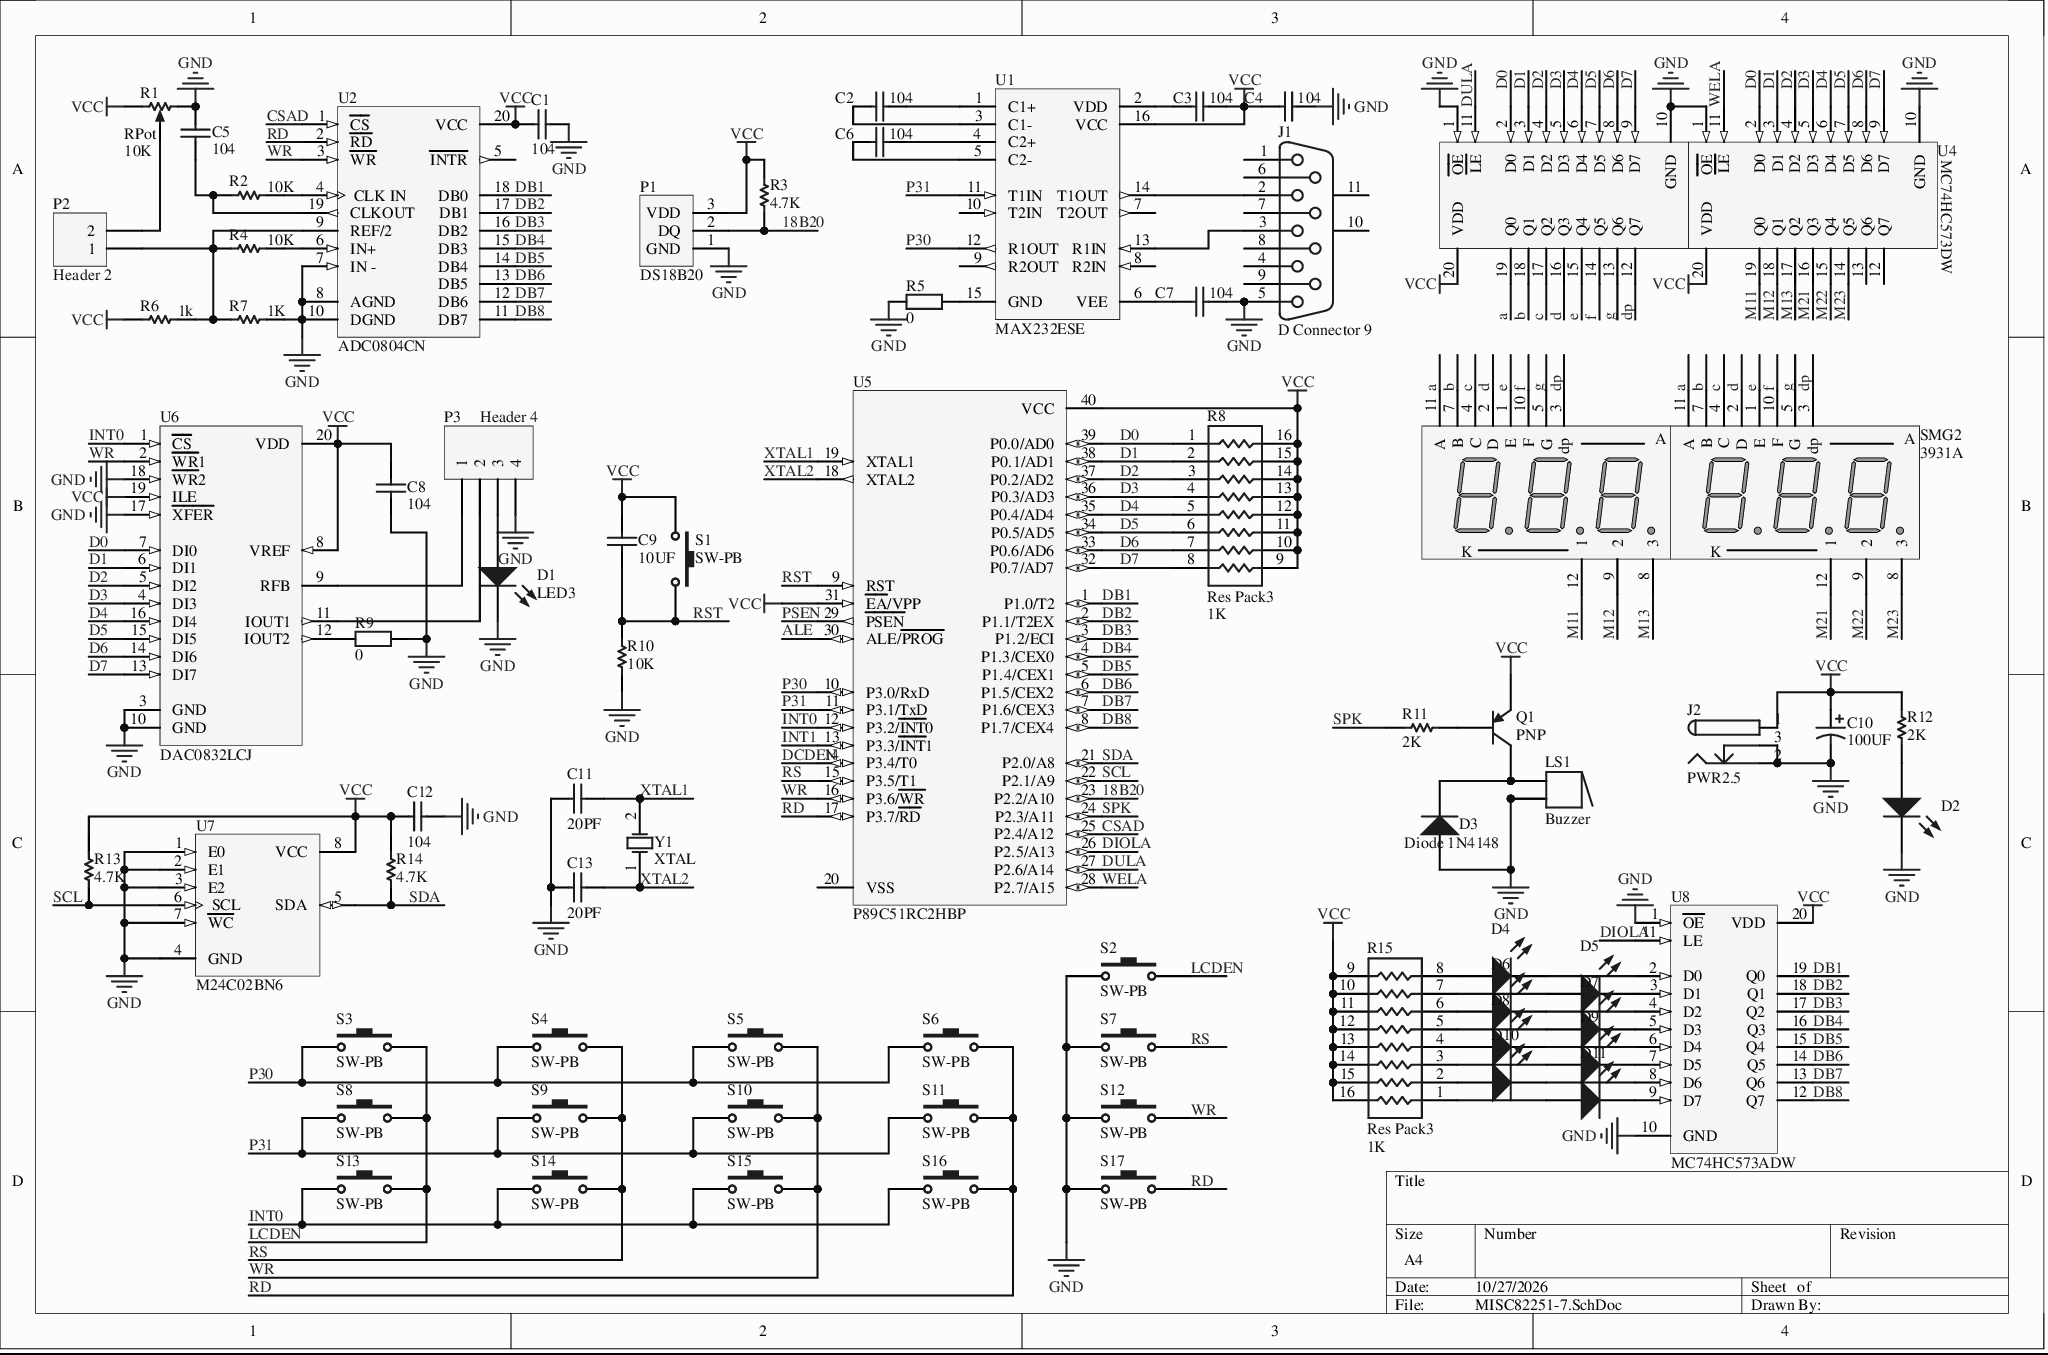
[diagram p0: MISC82251-7.SchDoc]
# Altium project MISC82251-3.PrjPcb
1 sheet, 74 parts. Net scope: global (net labels, ports and power ports of the same name join across sheets).
Board file: MISC82251.PcbDoc

## Sheet MISC82251-7.SchDoc
size A4

### Parts
C1  104  [RAD-0.3]
C2  104  [RAD-0.3]
C3  104  [RAD-0.3]
C4  104  [RAD-0.3]
C5  104  [RAD-0.3]
C6  104  [RAD-0.3]
C7  104  [RAD-0.3]
C8  104  [RAD-0.3]
C9  10UF  [RAD-0.3]
C10  100UF  [RB7.6-15]
C11  20PF  [RAD-0.1]
C12  104  [RAD-0.3]
C13  20PF  [RAD-0.1]
D1  LED3  [3.5X2.8X1.9]
D2  LED3  [3.5X2.8X1.9]  (value not drawn)
D3  Diode 1N4148  [DO-35]
D4  LED3  [3.5X2.8X1.9]  (value not drawn)
D5  LED3  [3.5X2.8X1.9]  (value not drawn)
D6  LED3  [3.5X2.8X1.9]  (value not drawn)
D7  LED3  [3.5X2.8X1.9]  (value not drawn)
D8  LED3  [3.5X2.8X1.9]  (value not drawn)
D9  LED3  [3.5X2.8X1.9]  (value not drawn)
D10  LED3  [3.5X2.8X1.9]  (value not drawn)
D11  LED3  [3.5X2.8X1.9]  (value not drawn)
J1  D Connector 9  [DSUB1.385-2H9]
J2  PWR2.5  [DC-002]
LS1  Buzzer  [ABSM-1574]
P1  DS18B20  [HDR1X3]
P2  Header 2  [HDR1X2]
P3  Header 4  [HDR1X4]
Q1  PNP  [SOT-23B_N]
R1  RPot  value 10K  [VR5]
R2  10K  [AXIAL-0.3]
R3  4.7K  [AXIAL-0.3]
R4  10K  [AXIAL-0.3]
R5  0  [AXIAL-0.4]
R6  1k  [AXIAL-0.3]
R7  1K  [AXIAL-0.3]
R8  Res Pack3  value 1K  [SO-16_N]
R9  0  [AXIAL-0.4]
R10  10K  [AXIAL-0.3]
R11  2K  [AXIAL-0.3]
R12  2K  [AXIAL-0.3]
R13  4.7K  [AXIAL-0.3]
R14  4.7K  [AXIAL-0.3]
R15  Res Pack3  value 1K  [SO-16_N]
S1  SW-PB  [SPST-2]
S2  SW-PB  [SPST-2]
S3  SW-PB  [SPST-2]
S4  SW-PB  [SPST-2]
S5  SW-PB  [SPST-2]
S6  SW-PB  [SPST-2]
S7  SW-PB  [SPST-2]
S8  SW-PB  [SPST-2]
S9  SW-PB  [SPST-2]
S10  SW-PB  [SPST-2]
S11  SW-PB  [SPST-2]
S12  SW-PB  [SPST-2]
S13  SW-PB  [SPST-2]
S14  SW-PB  [SPST-2]
S15  SW-PB  [SPST-2]
S16  SW-PB  [SPST-2]
S17  SW-PB  [SPST-2]
SMG1  3931A  [SMG 0.39-3P]
SMG2  3931A  [SMG 0.39-3P]
U1  MAX232ESE  [DIP16]
U2  ADC0804CN  [N020]
U3  MC74HC573DW  [751D-03]
U4  MC74HC573DW  [751D-03]
U5  P89C51RC2HBP  [SOT129-1]
U6  DAC0832LCJ  [J20A]
U7  M24C02BN6  [PSDIP8A]
U8  MC74HC573ADW  [751D-05]
Y1  XTAL  [R38]

### Nets
GND: C1.1 C4.1 C5.2 C7.1 C8.2 C10.2 C11.2 C12.2 C13.2 D1.2(K) D2.2(K) D3.1(A) J1.5 J2.2 J2.3 LS1.2 LS1.2A P1.1(GND) P3.4 R1.2(BOT) R5.1 R7.2 R9.2 R10.1 S2.1 S7.1 S12.1 S17.1 U2.7(IN_-) U2.8(AGND) U2.10(DGND) U3.1(~{OE}) U3.10(GND) U4.1(~{OE}) U4.10(GND) U6.3(GND) U6.10(GND) U6.17(~{XFER}) U6.18(~{WR}2) U7.1(E0) U7.2(E1) U7.3(E2) U7.4(GND) U7.7(~{WC}) U8.1(~{OE}) U8.10(GND)
VCC: C1.2 C3.1 C4.2 C8.1 C9.2 C10.1 C12.1 J2.1 P1.3(VDD) Q1.3(E) R1.1(TOP) R3.2 R6.1 R8.9 R8.10 R8.11 R8.12 R8.13 R8.14 R8.15 R8.16 R12.2 R13.2 R14.2 R15.9 R15.10 R15.11 R15.12 R15.13 R15.14 R15.15 R15.16 S1.1 U1.16(VCC) U2.20(VCC) U3.20(VDD) U4.20(VDD) U5.31(~{EA}/VPP) U5.40(VCC) U6.8(VREF) U6.19(ILE) U6.20(VDD) U7.8(VCC) U8.20(VDD)
18B20: P1.2(DQ) R3.1 U5.23(P2.2/A10)
a: SMG1.11(A) SMG2.11(A) U3.19(Q0)
ALE: U5.30(ALE/~{PROG})
b: SMG1.7(B) SMG2.7(B) U3.18(Q1)
c: SMG1.4(C) SMG2.4(C) U3.17(Q2)
CSAD: U2.1(~{CS}) U5.25(P2.4/A12)
d: SMG1.2(D) SMG2.2(D) U3.16(Q3)
D0: R8.1 U3.2(D0) U4.2(D0) U5.39(P0.0/AD0) U6.7(DI0)
D1: R8.2 U3.3(D1) U4.3(D1) U5.38(P0.1/AD1) U6.6(DI1)
D2: R8.3 U3.4(D2) U4.4(D2) U5.37(P0.2/AD2) U6.5(DI2)
D3: R8.4 U3.5(D3) U4.5(D3) U5.36(P0.3/AD3) U6.4(DI3)
D4: R8.5 U3.6(D4) U4.6(D4) U5.35(P0.4/AD4) U6.16(DI4)
D5: R8.6 U3.7(D5) U4.7(D5) U5.34(P0.5/AD5) U6.15(DI5)
D6: R8.7 U3.8(D6) U4.8(D6) U5.33(P0.6/AD6) U6.14(DI6)
D7: R8.8 U3.9(D7) U4.9(D7) U5.32(P0.7/AD7) U6.13(DI7)
DB1: U2.18(DB0) U5.1(P1.0/T2) U8.19(Q0)
DB2: U2.17(DB1) U5.2(P1.1/T2EX) U8.18(Q1)
DB3: U2.16(DB2) U5.3(P1.2/ECI) U8.17(Q2)
DB4: U2.15(DB3) U5.4(P1.3/CEX0) U8.16(Q3)
DB5: U2.14(DB4) U5.5(P1.4/CEX1) U8.15(Q4)
DB6: U2.13(DB5) U5.6(P1.5/CEX2) U8.14(Q5)
DB7: U2.12(DB6) U5.7(P1.6/CEX3) U8.13(Q6)
DB8: U2.11(DB7) U5.8(P1.7/CEX4) U8.12(Q7)
DCDEN: U5.14(P3.4/T0)
DIOLA: U5.26(P2.5/A13) U8.11(LE)
dp: SMG1.3(dp) SMG2.3(dp) U3.12(Q7)
DULA: U3.11(~{LE}) U5.27(P2.6/A14)
e: SMG1.1(E) SMG2.1(E) U3.15(Q4)
f: SMG1.10(F) SMG2.10(F) U3.14(Q5)
g: SMG1.5(G) SMG2.5(G) U3.13(Q6)
INT0: S13.1 S14.1 S15.1 S16.1 U5.12(P3.2/~{INT}0) U6.1(~{CS})
INT1: U5.13(P3.3/~{INT}1)
LCDEN: S2.2 S3.2 S8.2 S13.2
M11: SMG1.12(1) U4.19(Q0)
M12: SMG1.9(2) U4.18(Q1)
M13: SMG1.8(3) U4.17(Q2)
M21: SMG2.12(1) U4.16(Q3)
M22: SMG2.9(2) U4.15(Q4)
M23: SMG2.8(3) U4.14(Q5)
P30: S3.1 S4.1 S5.1 S6.1 U1.12(R1OUT) U5.10(P3.0/RxD)
P31: S8.1 S9.1 S10.1 S11.1 U1.11(T1IN) U5.11(P3.1/TxD)
PSEN: U5.29(~{PSEN})
RD: S6.2 S11.2 S16.2 S17.2 U2.2(~{RD}) U5.17(P3.7/~{RD})
RS: S4.2 S7.2 S9.2 S14.2 U5.15(P3.5/T1)
RST: C9.1 R10.2 S1.2 U5.9(RST)
SCL: R13.1 U5.22(P2.1/A9) U7.6(SCL)
SDA: R14.1 U5.21(P2.0/A8) U7.5(SDA)
SPK: R11.2 U5.24(P2.3/A11)
WELA: U4.11(~{LE}) U5.28(P2.7/A15)
WR: S5.2 S10.2 S12.2 S15.2 U2.3(~{WR}) U5.16(P3.6/~{WR}) U6.2(~{WR}1)
XTAL1: C11.1 U5.19(XTAL1) Y1.2(OSC2)
XTAL2: C13.1 U5.18(XTAL2) Y1.1(OSC1)
NetC2_1: C2.1 U1.1(C1+)
NetC2_2: C2.2 U1.3(C1-)
NetC3_2: C3.2 U1.2(VDD)
NetC5_1: C5.1 R2.1 U2.19(CLKOUT)
NetC6_1: C6.1 U1.4(C2+)
NetC6_2: C6.2 U1.5(C2-)
NetC7_2: C7.2 U1.6(VEE)
NetD1_1: D1.1(A) P3.3
NetD2_1: D2.1(A) R12.1
NetD3_2: D3.2(K) LS1.1 LS1.1A Q1.1(C)
NetD4_1: D4.1(A) R15.8
NetD4_2: D4.2(K) U8.2(D0)
NetD5_1: D5.1(A) R15.7
NetD5_2: D5.2(K) U8.3(D1)
NetD6_1: D6.1(A) R15.6
NetD6_2: D6.2(K) U8.4(D2)
NetD7_1: D7.1(A) R15.5
NetD7_2: D7.2(K) U8.5(D3)
NetD8_1: D8.1(A) R15.4
NetD8_2: D8.2(K) U8.6(D4)
NetD9_1: D9.1(A) R15.3
NetD9_2: D9.2(K) U8.7(D5)
NetD10_1: D10.1(A) R15.2
NetD10_2: D10.2(K) U8.8(D6)
NetD11_1: D11.1(A) R15.1
NetD11_2: D11.2(K) U8.9(D7)
NetJ1_2: J1.2 U1.14(T1OUT)
NetJ1_3: J1.3 U1.13(R1IN)
NetP2_1: P2.1 R4.1 R6.2 R7.1 U2.9(REF/2)
NetP2_2: P2.2 R1.3(TAP)
NetP3_1: P3.1 U6.9(RFB)
NetP3_2: P3.2 U6.11(IOUT1)
NetQ1_2: Q1.2(B) R11.1
NetR2_2: R2.2 U2.4(CLK_IN)
NetR4_2: R4.2 U2.6(IN+)
NetR5_2: R5.2 U1.15(GND)
NetR9_1: R9.1 U6.12(IOUT2)

Not connected (* = marked no-connect by the designer): J1 1 4 6 7 8 9 10(MH1) 11(MH2); U1 7(T2OUT) 8(R2IN)* 9(R2OUT) 10(T2IN)*; U2 5(~{INTR}); U4 12(Q7)* 13(Q6); U5 20(VSS)

### Library data of the parts
C1-C9 C11-C13 = Cap: Capacitor; Value: 100pF; Published: 8-Jun-2000; LatestRevisionDate: 17-Jul-2002; LatestRevisionNote: Re-released for DXP Platform.; PackageReference: RAD-0.3; PackageDescription: Radial Cap, Thru-Hole; 2 Leads; 0.3 in Pin Spacing; Publisher: Altium Limited
C10 = Cap Pol1: Polarized Capacitor (Radial); Value: 100pF; Published: 8-Jun-2000; LatestRevisionDate: 17-Jul-2002; LatestRevisionNote: Re-released for DXP Platform.; PackageReference: RB7.6-15; PackageDescription: Polarized Capacitor (Radial); 2 Leads; Publisher: Altium Limited
D1 D2 D4-D11 = LED3: Typical BLUE SiC LED; Published: 8-Jun-2000; LatestRevisionDate: 17-Dec-2003; LatestRevisionNote: PCB Footprint replaced.; DatasheetVersion: 16-Apr-2002; PackageVersion: 16-Apr-2002; PackageReference: 3.5X2.8X1.9; PackageDescription: SM LED; 2 C-Bend Leads; Body 3.5 x 2.8 x 1.9 mm, inc leads (LxWxH typ); Publisher: Altium Limited
D3 = Diode 1N4148: High Conductance Fast Diode; Published: 8-Jun-2000; LatestRevisionDate: 17-Jul-2002; LatestRevisionNote: Re-released for DXP Platform.; DatasheetVersion: 1997; PackageReference: DO-35; PackageDescription: Diode, Axial; Body 3.8 x 1.9 mm (LxDia. max), Lead Dia. 0.53 mm (max); Code_JEDEC: DO-204-AH; ComponentLink1Description: Manufacturer Link; ComponentLink2Description: Datasheet; ComponentLink2URL: http://www.fairchildsemi.com/ds/1N%2F1N4148.pdf; Publisher: Altium Limited
J1 = D Connector 9: Receptacle Assembly, 9 Position, Right Angle; PackageDocument: O; Positions: 9; Published: 15-Jun-2001; LatestRevisionDate: 17-Jul-2002; LatestRevisionNote: Re-released for DXP Platform.; DatasheetDocument: 1-Sep-1999; PackageReference: 788750; Orientation: Right Angle; Gender: Receptacle; Publisher: Altium Limited
J2 = DC_Socket
LS1 = Buzzer: Magnetic Transducer Buzzer; Published: 24-Mar-1999; LatestRevisionDate: 17-Dec-2003; LatestRevisionNote: Schematic revised, PCB Footprint replaced.; DatasheetVersion: 17-Dec-2003; PackageReference: ABSM-1574; PackageDescription: Magnetic Transducer Buzzer; ComponentLink1Description: Manufacturer Link; Publisher: Altium Limited
P1 = Header 3: Header, 3-Pin; LatestRevisionDate: 17-Jul-2002; LatestRevisionNote: Re-released for DXP Platform.; Publisher: Altium Limited
P2 = Header 2: Header, 2-Pin; LatestRevisionDate: 17-Jul-2002; LatestRevisionNote: Re-released for DXP Platform.; Publisher: Altium Limited
P3 = Header 4: Header, 4-Pin; LatestRevisionDate: 17-Jul-2002; LatestRevisionNote: Re-released for DXP Platform.; Publisher: Altium Limited
Q1 = PNP: PNP Bipolar Transistor; Published: 8-Jun-2000; LatestRevisionDate: 29-May-2009; LatestRevisionNote: IPC-7351 Footprint Added.; PackageVersion: Aug-1999; PackageReference: SOT-23B; PackageDescription: 3-Pin SOT-23 Package 0.95 mm Pitch, 2.4 mm Lead Span; Publisher: Altium Limited
R1 = RPot: Potentiometer; Sim Note: Enter the Resistance value and the set point into parameter fields.; Set Position: 0.5; Published: 8-Jun-2000; LatestRevisionDate: 17-Jul-2002; LatestRevisionNote: Re-released for DXP Platform.; PackageReference: VR5; PackageDescription: Variable Resistor, Thru-Hole; 3 Leads; Publisher: Altium Limited
R2-R4 R10-R14 = Res1: Resistor; Value: 1K; Published: 8-Jun-2000; LatestRevisionDate: 17-Jul-2002; LatestRevisionNote: Re-released for DXP Platform.; PackageReference: AXIAL-0.3; PackageDescription: Axial Device, Thru-Hole; 2 Leads; 0.3 in Pin Spacing; Publisher: Altium Limited
R5 R9 = Res2: Resistor; Value: 1K; Published: 8-Jun-2000; LatestRevisionDate: 17-Jul-2002; LatestRevisionNote: Re-released for DXP Platform.; PackageReference: AXIAL-0.4; PackageDescription: Axial Device, Thru-Hole; 2 Leads; 0.4 in Pin Spacing; Publisher: Altium Limited
R6 R7 = Res1: Resistor; Published: 8-Jun-2000; LatestRevisionDate: 17-Jul-2002; LatestRevisionNote: Re-released for DXP Platform.; PackageReference: AXIAL-0.3; PackageDescription: Axial Device, Thru-Hole; 2 Leads; 0.3 in Pin Spacing; Value: 1K; Publisher: Altium Limited
R8 R15 = Res Pack3: Isolated Resistor Network; Published: 24-Mar-1999; LatestRevisionDate: 29-May-2009; LatestRevisionNote: IPC-7351 Footprint Added.; PackageReference: SO-16; PackageDescription: 16-Pin Small Outline Integrated Circuit 1.27 mm Pitch; Code_JEDEC: MS-012-AC; Code_IPC: SOIC127P600-16; Publisher: Altium Limited
S1-S17 = SW-PB: Switch; Published: 24-Mar-1999; LatestRevisionDate: 17-Jul-2002; LatestRevisionNote: Re-released for DXP Platform.; PackageReference: SPST-2; PackageDescription: Switch; 2 Leads; Publisher: Altium Limited
SMG1 SMG2 = 3931A: 0.39 inch 3-digit common-cathode LED display; BOM名称: 0.39 inch 3-digit common-cathode
U1 = MAX232ESE: +5V Powered, Multi-Channel RS-232 Driver/Receiver; Code - JEDEC: MS-012-AC; Code - IPC: SO16; Published: 16-Jan-2001; Revision: 17-Jul-2002: Re-released for DXP Platform.; Package Reference: NSO16; Publisher: Altium Limited
U2 = ADC0804CN: 8-Bit Analog-to-Digital Converter with Differential Inputs; Package Information: Latest Revision: Oct-1995; Published: 15-Apr-2002; Datasheet: Linear Circuits Data Book 1989 Volume 2 (Oct-1988); Package Reference: N020; Publisher: Altium Limited
U3 U4 = MC74HC573DW: Octal 3-State Non-Inverting Transparent Latch; Published: 17-Jul-2002; Datasheet: High-Speed CMOS Logic Data, DL129 Rev4 (1989); Package Reference: 751D-03; Publisher: Altium Limited
U5 = P89C51RC2HBP: 80C51 8-Bit Flash Microcontroller Family, 32 kB ISP/IAP Flash with 512 B RAM.; Package Information: Latest Revision: Aug-2000; Code - JEDEC: MO-015; Published: 21-May-2003; Datasheet: Latest Revision: 24-May-2002; Package Reference: SOT129-1; Publisher: Altium Limited
U6 = DAC0832LCJ: 8-Bit uP-Compatible, Double-Buffered Digital-to-Analog Converter; Package Information: Latest Revision: 2000; Code - JEDEC: MS-015-AE; Published: 15-Apr-2002; Datasheet: Latest Revision: May-1999; Package Reference: J20A; Publisher: Altium Limited
U7 = M24C02BN6: 2Kbit Serial IIC Bus EEPROM; Package Information: Latest Revision: Jun-1998; Published: 24-Aug-2001; Revision: 17-Jul-2002: Re-released for DXP Platform.; Datasheet: Latest Revision: Sep-1999; Package Reference: PSDIP8A; Publisher: Altium Limited
U8 = MC74HC573ADW: Octal 3-State Non-Inverting Transparent Latch; Published: 15-Apr-2002; Datasheet: Latest Revision: Mar-2000; Package Reference: 751D-05; Publisher: Altium Limited
Y1 = XTAL: Crystal Oscillator; Published: 8-Jun-2000; LatestRevisionDate: 17-Jul-2002; LatestRevisionNote: Re-released for DXP Platform.; PackageReference: R38; PackageDescription: Crystal, Thru-Hole; 2 Leads; Body 3.1 x 8.2 mm (Dia.xH); Publisher: Altium Limited